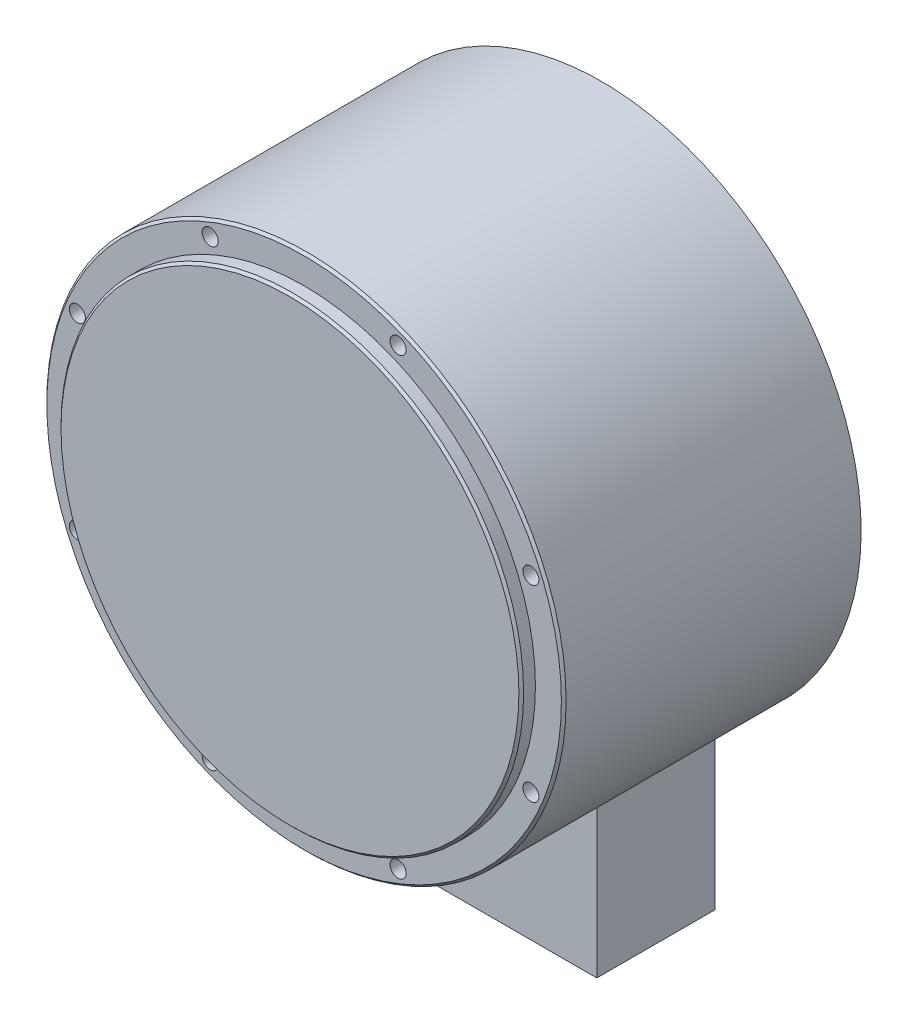
from build123d import *

# Parameters (mm, degrees)
SKETCH_1_R             = 110
EXTRUDE_1_DEPTH        = 126
SKETCH_2_R             = 98
EXTRUDE_2_DEPTH        = 6
SKETCH_3_W             = 96
SKETCH_3_H             = 71.025255747
EXTRUDE_3_DEPTH        = 50
CHAMFER_1_SIZE         = 1
HOLE_WIZARD_M8_1_D     = 6.8
HOLE_WIZARD_M8_1_DEPTH = 19.75
HOLE_WIZARD_M8_1_TIP   = 2.042926105
HOLE_WIZARD_M8_2_D     = 6.8
HOLE_WIZARD_M8_2_DEPTH = 19.75
HOLE_WIZARD_M8_2_TIP   = 2.042926105


with BuildPart() as part:
    # 草图1 → 凸台-拉伸1 (new body)
    with BuildSketch(Plane.XY):
        Circle(SKETCH_1_R)
    extrude(amount=EXTRUDE_1_DEPTH)

    # 草图2 → 凸台-拉伸2 (add)
    with BuildSketch(Plane.XY.offset(126)):
        Circle(SKETCH_2_R)
    extrude(amount=EXTRUDE_2_DEPTH)

    # 草图3 → 凸台-拉伸3 (add)
    with BuildSketch(Plane(origin=(0, 0, 0), x_dir=(-1, 0, 0), z_dir=(0, 0, -1))):
        with Locations((0, -134.487372127)):
            Rectangle(SKETCH_3_W, SKETCH_3_H)
    extrude(amount=-EXTRUDE_3_DEPTH)

    # 倒角1
    chamfer_1_edges = [part.edges().sort_by_distance(p)[0] for p in [
        (-110, 0, 126),
        (-98, 0, 132),
    ]]
    chamfer(chamfer_1_edges, length=CHAMFER_1_SIZE)

    # M8 螺纹孔1
    with Locations(Plane(origin=(0, 0, 0), x_dir=(-1, 0, 0), z_dir=(0, 0, -1))):
        with Locations((0, 115), (81.317279836, 81.317279836), (115, 0), (81.317279836, -81.317279836), (0, -115), (-81.317279836, -81.317279836), (-115, 0), (-81.317279836, 81.317279836)):
            Hole(HOLE_WIZARD_M8_1_D / 2, depth=HOLE_WIZARD_M8_1_DEPTH)
            with Locations((0, 0, -(HOLE_WIZARD_M8_1_DEPTH + HOLE_WIZARD_M8_1_TIP / 2))):  # 118° drill point
                Cone(0, HOLE_WIZARD_M8_1_D / 2, HOLE_WIZARD_M8_1_TIP, mode=Mode.SUBTRACT)

    # M8 螺纹孔2
    with Locations(Plane.XY.offset(132)):
        with Locations((39.799076966, 96.083471381), (96.083471381, 39.799076966), (96.083471381, -39.799076966), (39.799076966, -96.083471381), (-39.799076966, -96.083471381), (-96.083471381, -39.799076966), (-96.083471381, 39.799076966), (-39.799076966, 96.083471381)):
            Hole(HOLE_WIZARD_M8_2_D / 2, depth=HOLE_WIZARD_M8_2_DEPTH)
            with Locations((0, 0, -(HOLE_WIZARD_M8_2_DEPTH + HOLE_WIZARD_M8_2_TIP / 2))):  # 118° drill point
                Cone(0, HOLE_WIZARD_M8_2_D / 2, HOLE_WIZARD_M8_2_TIP, mode=Mode.SUBTRACT)


solid = part.part
